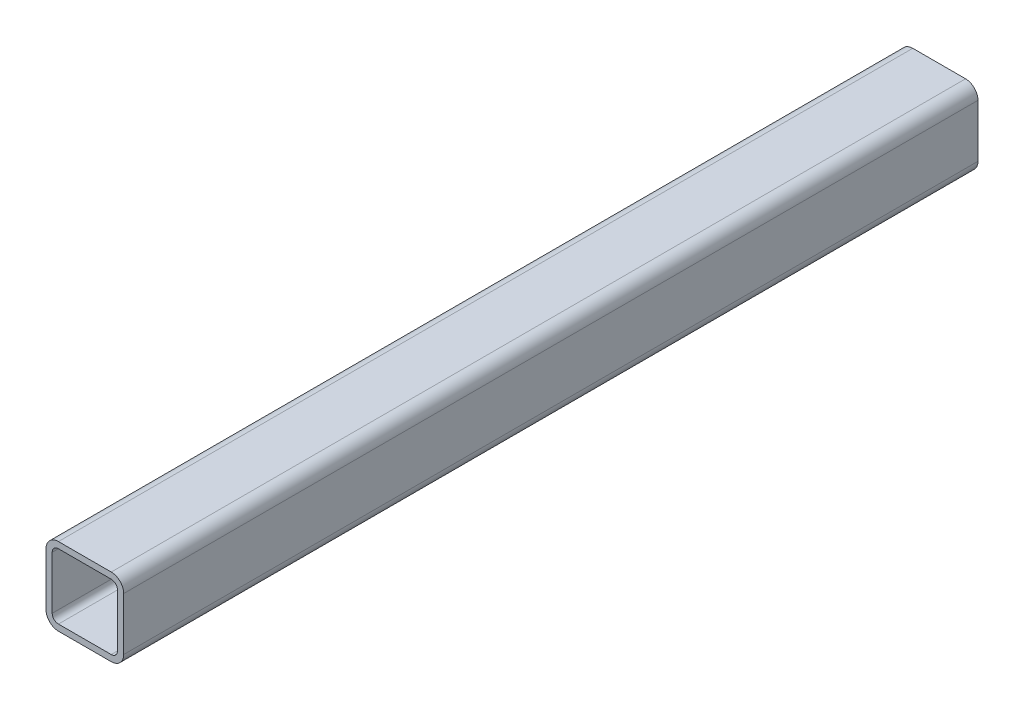
SolidWorks part; units mm, degrees
material "AISI 1045 钢，冷拔"
ref_plane "Front Plane" through (0, 0, 0) normal (0, 0, 1) x (1, 0, 0)
ref_plane "Top Plane" through (0, 0, 0) normal (0, 1, 0) x (1, 0, 0)
ref_plane "Right Plane" through (0, 0, 0) normal (1, 0, 0) x (0, 0, -1)
sketch "Sketch1" plane through (0, 0, 0) normal (0, 0, 1) x (1, 0, 0)
  line L0 (-21.0947, 0) -> (28.2454, 0) construction
  line L1 (0, 28.305) -> (0, -28.2454) construction
  line L2 (-17, 21) -> (17, 21)
  line L3 (-17, -25) -> (17, -25)
  line L4 (-25, -17) -> (-25, 17)
  line L5 (-17, 25) -> (17, 25)
  line L6 (25, -17) -> (25, 17)
  line L7 (-25, -25) -> (25, 25) construction
  line L8 (-25, 25) -> (25, -25) construction
  line L9 (21, -17) -> (21, 17)
  line L10 (-17, -21) -> (17, -21)
  line L11 (-21, -17) -> (-21, 17)
  arc A0 (17, -25) -> (25, -17) centre (17, -17) ccw
  arc A1 (-17, -25) -> (-25, -17) centre (-17, -17) cw
  arc A2 (17, 25) -> (25, 17) centre (17, 17) cw
  arc A3 (-25, 17) -> (-17, 25) centre (-17, 17) cw
  arc A4 (-21, 17) -> (-17, 21) centre (-17, 17) cw
  arc A5 (17, 21) -> (21, 17) centre (17, 17) cw
  arc A6 (17, -21) -> (21, -17) centre (17, -17) ccw
  arc A7 (-17, -21) -> (-21, -17) centre (-17, -17) cw
  point P5 (0, 0)
  dimension "D3" = 8
  dimension "D1" = 50
  dimension "D2" = 50
  dimension "D4" = 4
extrude "Boss-Extrude1" add sketch "Sketch1" along normal mid plane 550
